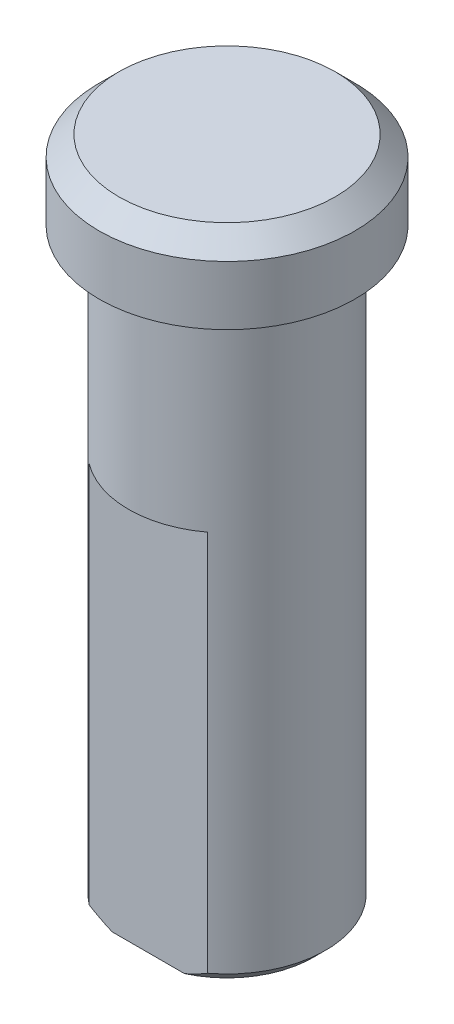
from build123d import *

# Parameters (mm, degrees)
SKETCH1_R           = 2.5
BOSS_EXTRUDE1_DEPTH = 15
SKETCH2_R           = 3.25
BOSS_EXTRUDE2_DEPTH = 2
CHAMFER1_SIZE       = 0.5
CHAMFER2_SIZE       = 0.3
SKETCH3_W           = 5.914103074
SKETCH3_H           = 1
CUT_EXTRUDE1_DEPTH  = 10


with BuildPart() as part:
    # Sketch1 → Boss-Extrude1 (new body)
    with BuildSketch(Plane(origin=(0, 0, 0), x_dir=(1, 0, 0), z_dir=(0, 1, 0))):
        with Locations(Location((0, 0, 0), (0, 0, 270))):
            Circle(SKETCH1_R)
    extrude(amount=BOSS_EXTRUDE1_DEPTH)

    # Sketch2 → Boss-Extrude2 (add)
    with BuildSketch(Plane(origin=(0, 15, 0), x_dir=(1, 0, 0), z_dir=(0, 1, 0))):
        with Locations(Location((0, 0, 0), (0, 0, 270))):
            Circle(SKETCH2_R)
    extrude(amount=BOSS_EXTRUDE2_DEPTH)

    # Chamfer1
    chamfer1_edges = [part.edges().sort_by_distance(p)[0] for p in [
        (0, 17, -3.25),
    ]]
    chamfer(chamfer1_edges, length=CHAMFER1_SIZE)

    # Chamfer2
    chamfer2_edges = [part.edges().sort_by_distance(p)[0] for p in [
        (0, 0, -2.5),
    ]]
    chamfer(chamfer2_edges, length=CHAMFER2_SIZE)

    # Sketch3 → Cut-Extrude1 (cut)
    with BuildSketch(Plane.XZ):
        with Locations((0, 2.5)):
            Rectangle(SKETCH3_W, SKETCH3_H)
    extrude(amount=-CUT_EXTRUDE1_DEPTH, mode=Mode.SUBTRACT)


solid = part.part
